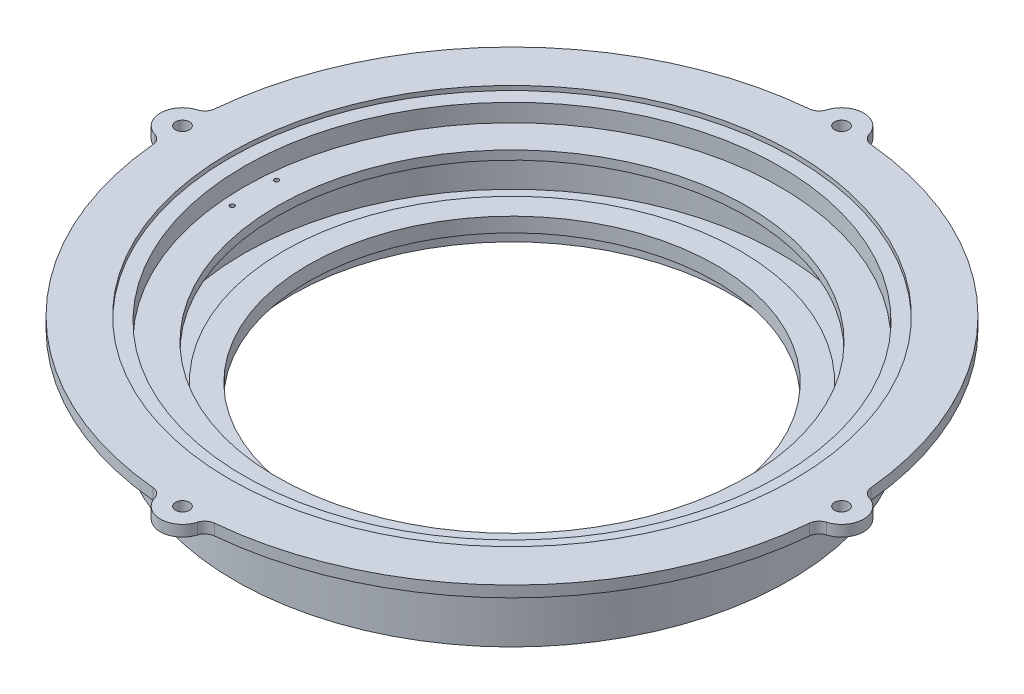
from build123d import *

# Parameters (mm, degrees)
SKETCH2_R           = 127.5
CUT_EXTRUDE1_DEPTH  = 2
SKETCH3_R           = 10
BOSS_EXTRUDE1_DEPTH = 5
FILLET1_R           = 5
SKETCH4_R           = 3.15
CUT_EXTRUDE2_DEPTH  = 10
FILLET2_R           = 7.5
SKETCH5_R           = 1
CUT_EXTRUDE3_DEPTH  = 5


with BuildPart() as part:
    # Sketch1 → Revolve1 (revolve)
    with BuildSketch(Plane.XY):
        Polygon((-125, 139.5), (-125, 175.5), (-148.746139417, 175.5), (-148.746139417, 180.5), (-121, 180.5), (-121, 170.5), (-106, 170.5), (-106, 166.5), (-121, 166.5), (-121, 144.5), (-103, 144.5), (-103, 154.5), (-92, 154.5), (-92, 147.962623379), (-99, 147.962623379), (-99, 139.5), align=None)
    revolve(axis=Axis((0, 0, 0), (0, -1, 0)))

    # Sketch2 → Cut-Extrude1 (cut)
    with BuildSketch(Plane(origin=(0, 180.5, 0), x_dir=(1, 0, 0), z_dir=(0, 1, 0))):
        with Locations(Location((0, 0, 0), (0, 0, 180))):
            Circle(SKETCH2_R)
    extrude(amount=-CUT_EXTRUDE1_DEPTH, mode=Mode.SUBTRACT)

    # Sketch3 → Boss-Extrude1 (add)
    with BuildSketch(Plane.XZ.offset(-175.5)):
        with Locations((0, -148.746139417)):
            Circle(SKETCH3_R)
        with Locations((-148.746139417, 0)):
            Circle(SKETCH3_R)
        with Locations((0, 148.746139417)):
            Circle(SKETCH3_R)
        with Locations((148.746139417, 0)):
            Circle(SKETCH3_R)
    extrude(amount=-BOSS_EXTRUDE1_DEPTH)

    # Fillet1
    fillet1_edges = [part.edges().sort_by_distance(p)[0] for p in [
        (-9.994348791, 178, -148.409996239),
        (9.994348791, 178, -148.409996239),
        (-148.409996239, 178, 9.994348791),
        (-148.409996239, 178, -9.994348791),
        (9.994348791, 178, 148.409996239),
        (-9.994348791, 178, 148.409996239),
        (148.409996239, 178, -9.994348791),
        (148.409996239, 178, 9.994348791),
    ]]
    fillet(fillet1_edges, radius=FILLET1_R)

    # Sketch4 → Cut-Extrude2 (cut)
    with BuildSketch(Plane.XZ.offset(-175.5)):
        with Locations((148.746139417, 0)):
            Circle(SKETCH4_R)
        with Locations((0, -148.746139417)):
            Circle(SKETCH4_R)
        with Locations((-148.746139417, 0)):
            Circle(SKETCH4_R)
        with Locations((0, 148.746139417)):
            Circle(SKETCH4_R)
    extrude(amount=-CUT_EXTRUDE2_DEPTH, mode=Mode.SUBTRACT)

    # Fillet2
    fillet2_edges = [part.edges().sort_by_distance(p)[0] for p in [
        (125, 175.5, 0),
    ]]
    fillet(fillet2_edges, radius=FILLET2_R)

    # Sketch5 → Cut-Extrude3 (cut)
    with BuildSketch(Plane(origin=(0, 170.5, 0), x_dir=(1, 0, 0), z_dir=(0, 1, 0))):
        with Locations(Location((-116.275298476, 10, 0), (0, 0, 180))):
            Circle(SKETCH5_R)
        with Locations(Location((-116.275298476, -10, 0), (0, 0, 180))):
            Circle(SKETCH5_R)
        with Locations(Location((116.275298476, 10, 0), (0, 0, 180))):
            Circle(SKETCH5_R)
        with Locations(Location((116.275298476, -10, 0), (0, 0, 180))):
            Circle(SKETCH5_R)
    extrude(amount=-CUT_EXTRUDE3_DEPTH, mode=Mode.SUBTRACT)


solid = part.part
